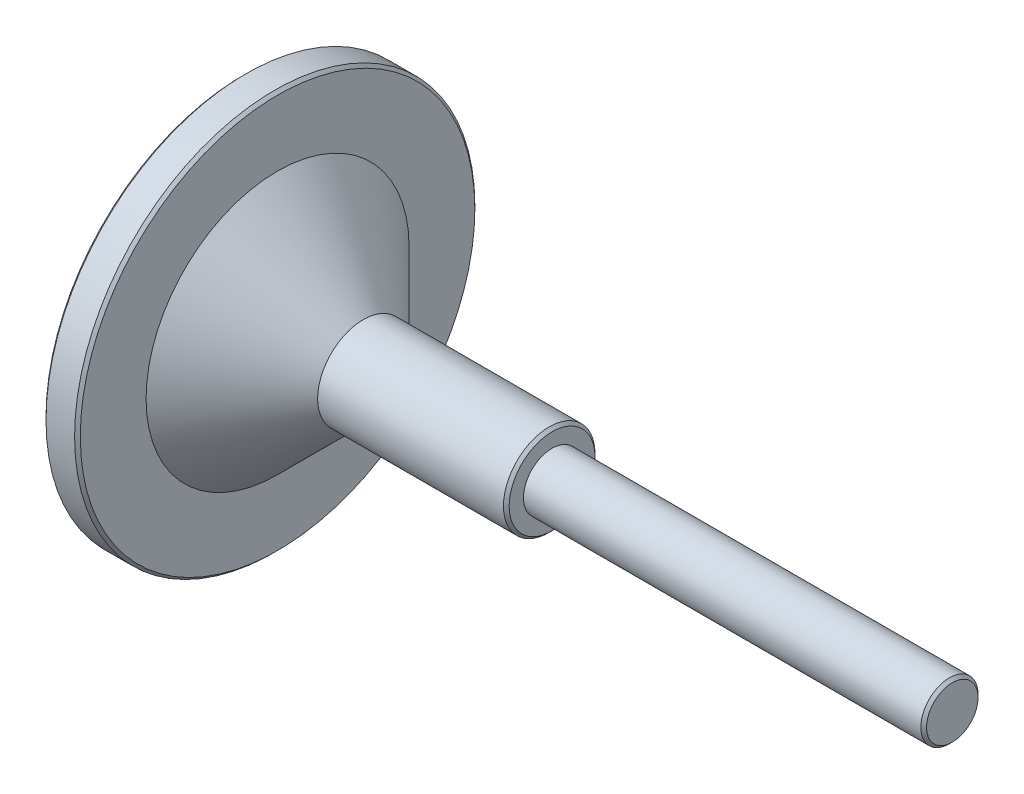
from build123d import *

# Parameters (mm, degrees)
CHAMFER1_SIZE = 0.5
CHAMFER2_SIZE = 0.5
CHAMFER3_SIZE = 15


with BuildPart() as part:
    # Sketch1 → Revolve1 (revolve)
    with BuildSketch(Plane.XY, mode=Mode.PRIVATE) as revolve1_sk:
        Polygon((0, 0), (0, 35), (6, 35), (6, 8), (54, 8), (54, 5), (124, 5), (124, 0), align=None)
    revolve(revolve1_sk.sketch.rotate(Axis((0, 0, 0), (1, 0, 0)), 90), axis=Axis((0, 0, 0), (1, 0, 0)))

    # Chamfer1
    chamfer1_edges = [part.edges().sort_by_distance(p)[0] for p in [
        (54, 0, -8),
        (6, 0, -35),
        (0, 0, -35),
    ]]
    chamfer(chamfer1_edges, length=CHAMFER1_SIZE)

    # Chamfer2
    chamfer2_edges = [part.edges().sort_by_distance(p)[0] for p in [
        (124, 0, -5),
    ]]
    chamfer(chamfer2_edges, length=CHAMFER2_SIZE)

    # Chamfer3
    chamfer3_edges = [part.edges().sort_by_distance(p)[0] for p in [
        (6, 0, -8),
    ]]
    chamfer(chamfer3_edges, length=CHAMFER3_SIZE)


solid = part.part
